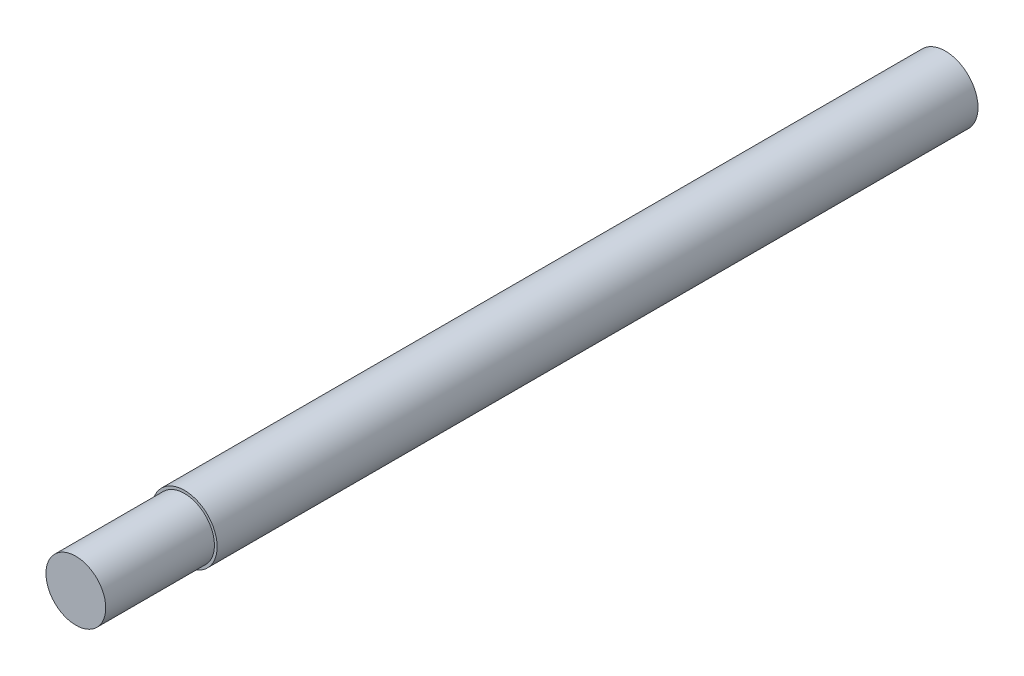
from build123d import *

# Parameters (mm, degrees)
SKETCH_1_R          = 6
EXTRUDE_3_DEPTH     = 80
SKETCH_3_R          = 6
SKETCH_3_R_2        = 5.5
CUT_EXTRUDE_1_DEPTH = 20


with BuildPart() as part:
    # 草图1 → 凸台-拉伸3 (new, symmetric)
    with BuildSketch(Plane.XY):
        Circle(SKETCH_1_R)
    extrude(amount=EXTRUDE_3_DEPTH, both=True)

    # 草图3 → 切除-拉伸1 (cut)
    with BuildSketch(Plane.XY.offset(80)):
        Circle(SKETCH_3_R)
        Circle(SKETCH_3_R_2, mode=Mode.SUBTRACT)
    extrude(amount=-CUT_EXTRUDE_1_DEPTH, mode=Mode.SUBTRACT)


solid = part.part
